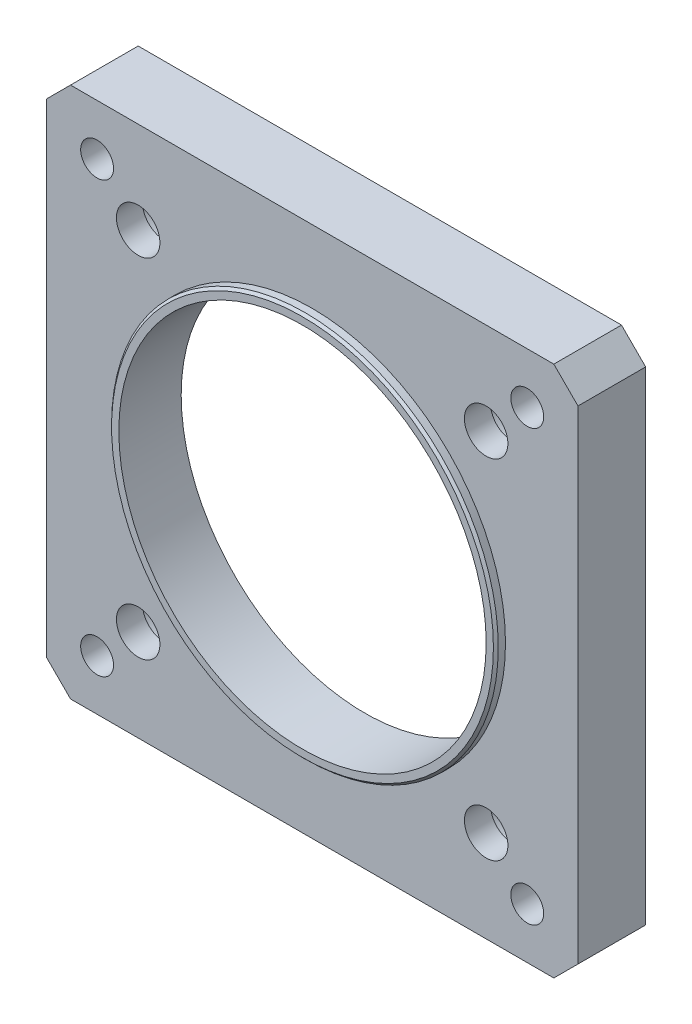
SolidWorks part; units mm, degrees
material "6061Al"
ref_plane "前视基准面" through (0, 0, 0) normal (0, 0, 1) x (1, 0, 0)
ref_plane "上视基准面" through (0, 0, 0) normal (0, 1, 0) x (1, 0, 0)
ref_plane "右视基准面" through (0, 0, 0) normal (1, 0, 0) x (0, 0, -1)
sketch "草图1" plane through (0, 0, 0) normal (0, 0, 1) x (1, 0, 0)
  line L1 (-55, -55) -> (55, -55)
  line L2 (-55, -55) -> (-55, 55)
  line L3 (-55, 55) -> (55, 55)
  line L4 (55, -55) -> (55, 55)
  line L5 (-55, -55) -> (55, 55) construction
  line L6 (-55, 55) -> (55, -55) construction
  point P0 (0, 0)
  dimension "D1" = 110
extrude "凸台-拉伸1" add sketch "草图1" along normal blind 14
sketch "草图2" plane through (0, 0, 14) normal (0, 0, 1) x (1, 0, 0)
  circle A0 centre (0, 0) radius 40
  circle A1 centre (0, 0) radius 38
  dimension "D1" = 80
  dimension "D2" = 2
extrude "凸台-拉伸2" add sketch "草图2" along normal blind 2
sketch "草图3" plane through (0, 0, 14) normal (0, 0, 1) x (1, 0, 0)
  circle A1 centre (0, 0) radius 38
  circle A2 centre (0, 0) radius 38
  dimension "D1" = 0
extrude "切除-拉伸1" cut sketch "草图3" against normal through all
sketch "草图4" plane through (0, 0, 0) normal (0, 0, -1) x (-1, 0, 0)
  circle A0 centre (0, 0) radius 42.5
  dimension "D1" = 85
extrude "切除-拉伸2" cut sketch "草图4" against normal blind 3.1
hole_wizard "M8 螺纹孔1" positions "草图5" profile "草图6" tap size "M8" standard "ISO" end condition through all
sketch "草图5" plane through (0, 0, 0) normal (0, 0, -1) x (-1, 0, 0)
  line L1 (-44.5, -44.5) -> (44.5, -44.5)
  line L2 (-44.5, -44.5) -> (-44.5, 44.5)
  line L3 (-44.5, 44.5) -> (44.5, 44.5)
  line L4 (44.5, -44.5) -> (44.5, 44.5)
  line L5 (-44.5, -44.5) -> (44.5, 44.5) construction
  line L6 (-44.5, 44.5) -> (44.5, -44.5) construction
  point P0 (-44.5, 44.5)
  point P3 (0, 0)
  point P4 (44.5, 44.5)
  point P7 (-44.5, -44.5)
  point P9 (44.5, -44.5)
  dimension "D1" = 89
sketch "草图6" plane through (44.5, 44.5, 0) normal (1, 0, 0) x (0, 1, 0)
  line L0 (0, 0) -> (0, 16)
  line L1 (0, 16) -> (3.4, 16)
  line L2 (3.4, 16) -> (3.4, 0)
  line L5 (3.4, 0) -> (0, 0)
  line L11 (0, -6.35) -> (0, 107.95) construction
  dimension "通孔螺纹孔钻头直径" = 6.8
  dimension "通孔螺纹孔钻头深度" = 16
cosmetic thread "孔螺蚊线1" parameters "D2"=8
cosmetic thread "孔螺蚊线2" parameters "D2"=8
cosmetic thread "孔螺蚊线3" parameters "D2"=8
cosmetic thread "孔螺蚊线4" parameters "D2"=8
hole_wizard "M8 六角凹头螺钉的柱形沉头孔1" positions "草图7" profile "草图8" counterbore size "M8" standard "ISO" end condition through all
sketch "草图7" plane through (0, 0, 0) normal (0, 0, -1) x (-1, 0, 0)
  line L3 (0, 0) -> (77.5022, 0) construction
  line L7 (-36, -36) -> (36, -36)
  line L8 (-36, -36) -> (-36, 36)
  line L9 (-36, 36) -> (36, 36)
  line L10 (36, -36) -> (36, 36)
  line L11 (-36, -36) -> (36, 36) construction
  line L12 (-36, 36) -> (36, -36) construction
  point P29 (36, 36)
  point P32 (-36, -36)
  point P33 (-36, 36)
  point P34 (36, -36)
  dimension "D1" = 72
sketch "草图8" plane through (-36, -36, 0) normal (1, 0, 0) x (0, 1, 0)
  line L0 (0, 0) -> (0, 16)
  line L1 (0, 16) -> (4.5, 16)
  line L3 (4.5, 16) -> (4.5, 8.6)
  line L4 (4.5, 8.6) -> (7.5, 8.6)
  line L5 (7.5, 8.6) -> (7.5, 0)
  line L7 (7.5, 0) -> (0, 0)
  line L11 (0, -6.35) -> (0, 107.95) construction
  dimension "通孔孔直径" = 9
  dimension "通孔孔深度" = 16
  dimension "柱形沉头孔直径" = 15
  dimension "柱形沉头孔深度" = 8.6
chamfer "倒角1" distance 5 angle 45 4 edges at (55, -55, 7) (-55, -55, 7) (-55, 55, 7) (55, 55, 7)
chamfer "倒角2" distance 0.5 angle 45 2 edges at (40, 0, 16) (-42.5, 0, 0)
